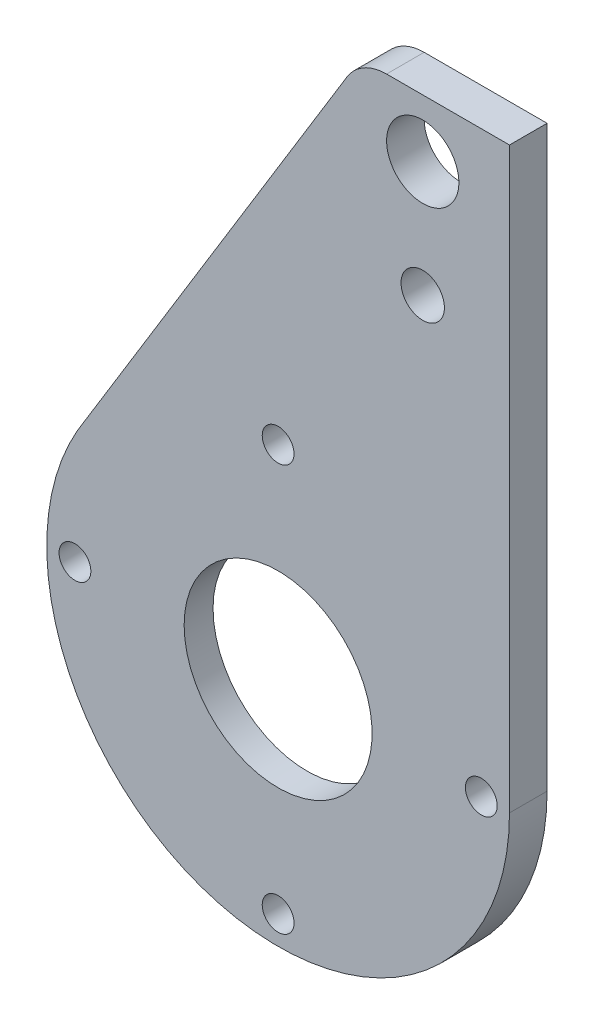
from build123d import *

# Parameters (mm, degrees)
SKETCH_1_R          = 32.5
SKETCH_1_R_2        = 12.5
SKETCH_1_R_3        = 7.5
EXTRUDE_1_DEPTH     = 13
CUT_EXTRUDE_START   = 3
SKETCH_2_R          = 60.5
CUT_EXTRUDE_2_DEPTH = 219.79851714
SKETCH_4_R          = 5.5
CUT_EXTRUDE_3_DEPTH = 216.79851714


with BuildPart() as part:
    # 草图1 → 凸台-拉伸1 (new body)
    with BuildSketch(Plane.XY):
        with BuildLine():
            Line((80, 200), (37.5, 200))
            ThreePointArc((37.5, 200), (29.674290769, 197.955582218), (23.848458927, 192.34478438))
            Line((23.848458927, 192.34478438), (-69.388730207, 39.814621941))
            ThreePointArc((-69.388730207, 39.814621941), (-20.602203565, -77.30167662), (80, 0))
            Line((80, 0), (80, 160))
            Line((80, 160), (80, 200))
        make_face()
        with Locations(Location((0, 0, 0), (0, 0, 180))):
            Circle(SKETCH_1_R, mode=Mode.SUBTRACT)
        with Locations(Location((50, 180, 0), (0, 0, 180))):
            Circle(SKETCH_1_R_2, mode=Mode.SUBTRACT)
        with Locations(Location((50, 140, 0), (0, 0, 180))):
            Circle(SKETCH_1_R_3, mode=Mode.SUBTRACT)
    extrude(amount=EXTRUDE_1_DEPTH)

    # 草图2 → 切除-拉伸2 (cut, through all)
    with BuildSketch(Plane.XY.offset(CUT_EXTRUDE_START)):
        Circle(SKETCH_2_R)
    extrude(amount=-CUT_EXTRUDE_2_DEPTH, mode=Mode.SUBTRACT)

    # 草图4 → 切除-拉伸3 (cut, through all)
    with BuildSketch(Plane(origin=(0, 0, 0), x_dir=(-1, 0, 0), z_dir=(0, 0, -1))):
        with Locations((70.25, 0)):
            Circle(SKETCH_4_R)
        with Locations((0, -70.25)):
            Circle(SKETCH_4_R)
        with Locations((-70.25, 0)):
            Circle(SKETCH_4_R)
        with Locations((0, 70.25)):
            Circle(SKETCH_4_R)
    extrude(amount=-CUT_EXTRUDE_3_DEPTH, mode=Mode.SUBTRACT)


solid = part.part
